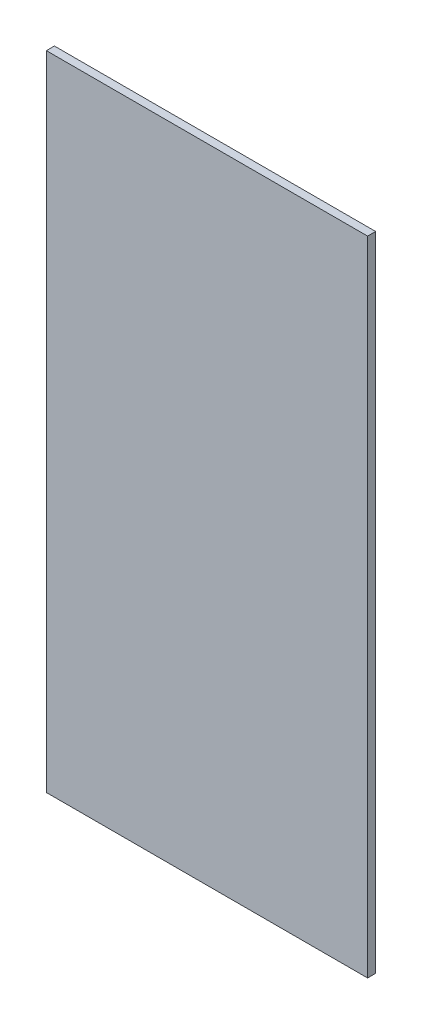
SolidWorks part; units mm, degrees
material "标准件"
ref_plane "前视基准面" through (0, 0, 0) normal (0, 0, 1) x (1, 0, 0)
ref_plane "上视基准面" through (0, 0, 0) normal (0, 1, 0) x (1, 0, 0)
ref_plane "右视基准面" through (0, 0, 0) normal (1, 0, 0) x (0, 0, -1)
sketch "草图1" plane through (0, 0, 0) normal (0, 0, 1) x (1, 0, 0)
  line L1 (-20, -40) -> (20, -40)
  line L2 (-20, -40) -> (-20, 40)
  line L3 (-20, 40) -> (20, 40)
  line L4 (20, -40) -> (20, 40)
  line L5 (-20, -40) -> (20, 40) construction
  line L6 (-20, 40) -> (20, -40) construction
  point P0 (0, 0)
  dimension "D1" = 40
  dimension "D2" = 80
extrude "凸台-拉伸1" add sketch "草图1" along normal mid plane 1
